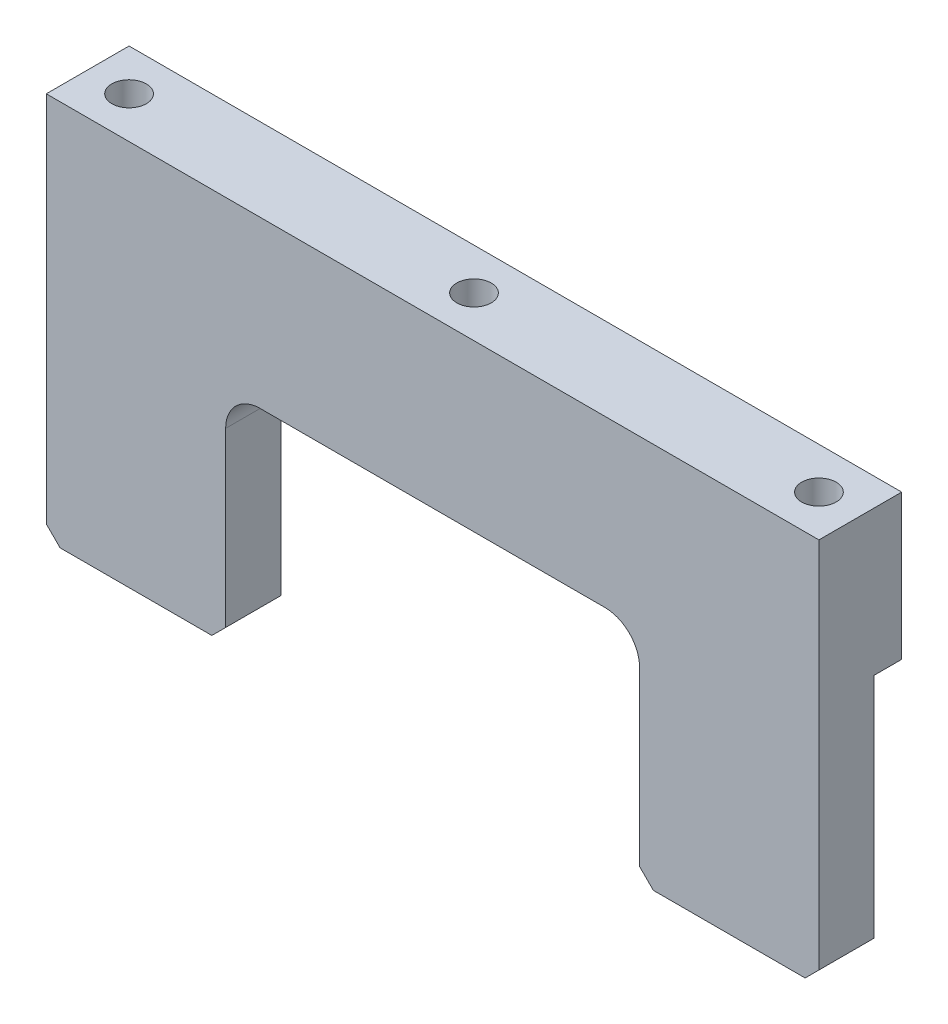
SolidWorks part; units mm, degrees
material "AL6061"
ref_plane "Front Plane" through (0, 0, 0) normal (0, 0, 1) x (1, 0, 0)
ref_plane "Top Plane" through (0, 0, 0) normal (0, 1, 0) x (1, 0, 0)
ref_plane "Right Plane" through (0, 0, 0) normal (1, 0, 0) x (0, 0, -1)
sketch "Sketch1" plane through (0, 0, 0) normal (0, 0, 1) x (1, 0, 0)
  line L1 (0, 0) -> (112, 0)
  line L2 (0, 0) -> (0, 56)
  line L3 (0, 56) -> (112, 56)
  line L4 (112, 0) -> (112, 56)
  dimension "D1" = 112
  dimension "D2" = 56
extrude "Boss-Extrude1" add sketch "Sketch1" along normal blind 12
sketch "Sketch2" plane through (0, 0, 0) normal (0, 0, -1) x (-1, 0, 0)
  line L0 (0, 56) -> (0, 0) construction
  line L1 (-112, 0) -> (0, 0)
  line L2 (-112, 0) -> (-112, 35)
  line L3 (-112, 35) -> (0, 35)
  line L4 (0, 0) -> (0, 35)
  dimension "D1" = 35
extrude "Cut-Extrude1" cut sketch "Sketch2" against normal blind 4
hole_wizard "M6 Tapped Hole1" positions "Sketch5" profile "Sketch4" tap size "M6" standard "ISO"
sketch "Sketch5" plane through (0, 56, 0) normal (0, 1, 0) x (1, 0, 0)
  line L0 (0, -6) -> (112, -6) construction
  line L1 (0, -12) -> (0, 0) construction
  line L2 (112, -12) -> (112, 0) construction
  line L5 (56, 0) -> (56, -12) construction
  line L6 (112, 0) -> (0, 0) construction
  line L7 (112, -12) -> (0, -12) construction
  point P18 (6, -6)
  point P20 (56, -6)
  point P23 (106, -6)
  dimension "D1" = 100
sketch "Sketch4" plane through (106, 56, 6) normal (1, 0, 0) x (0, 0, 1)
  line L0 (0, 0) -> (0, 16.5022)
  line L1 (0, 16.5022) -> (2.5, 15)
  line L2 (2.5, 15) -> (2.5, 0)
  line L5 (2.5, 0) -> (0, 0)
  line L10 (0, 16.5022) -> (-2.5, 15) construction
  line L11 (0, -6.35) -> (0, 107.95) construction
  dimension "螺纹孔钻头直径" = 5
  dimension "螺纹孔钻头深度" = 15
  dimension "导头角度" = 118
cosmetic thread "Cosmetic thread 1" parameters "D1"=12, "D2"=6
cosmetic thread "Cosmetic thread 2" parameters "D1"=12, "D2"=6
cosmetic thread "Cosmetic thread 3" parameters "D1"=12, "D2"=6
sketch "Sketch6" plane through (0, 0, 4) normal (0, 0, -1) x (-1, 0, 0)
  line L0 (-56, 56) -> (-56, 0) construction
  line L1 (-112, 56) -> (0, 56) construction
  line L2 (-112, 0) -> (0, 0) construction
  line L4 (-86, 0) -> (-26, 0)
  line L5 (-86, 0) -> (-86, 32)
  line L6 (-86, 32) -> (-26, 32)
  line L7 (-26, 0) -> (-26, 32)
  dimension "D1" = 32
  dimension "D2" = 60
extrude "Cut-Extrude2" cut sketch "Sketch6" against normal through all
fillet "Fillet1" radius 5 2 edges at (26, 32, 8) (86, 32, 8)
chamfer "Chamfer1" distance 2 angle 45 4 edges at (0, 0, 8) (26, 0, 8) (86, 0, 8) (112, 0, 8)
